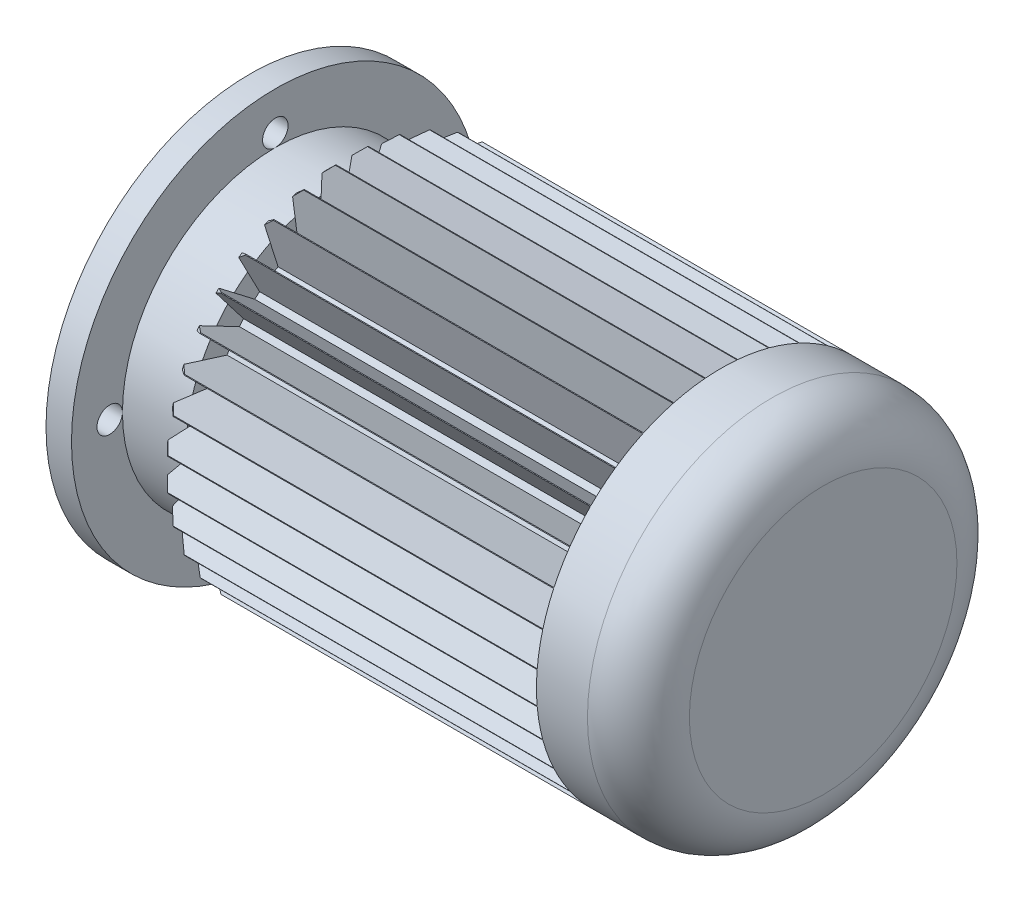
SolidWorks part; units mm, degrees
ref_plane "前视基准面" through (0, 0, 0) normal (0, 0, 1) x (1, 0, 0)
ref_plane "上视基准面" through (0, 0, 0) normal (0, 1, 0) x (1, 0, 0)
ref_plane "右视基准面" through (0, 0, 0) normal (1, 0, 0) x (0, 0, -1)
sketch "草图1" plane through (0, 0, 0) normal (0, 0, 1) x (1, 0, 0)
  line L0 (0, 0) -> (197.0687, 0) construction
  line L1 (0, 0) -> (0, 55)
  line L2 (0, -55) -> (0, 55) construction
  line L3 (0, 55) -> (3.5, 55)
  line L4 (3.5, 55) -> (3.5, 80)
  line L5 (3.5, 80) -> (13.5, 80)
  line L6 (13.5, 80) -> (13.5, 60)
  line L7 (13.5, 60) -> (38.5, 60)
  line L8 (38.5, 60) -> (38.5, 72.5)
  line L9 (38.5, 72.5) -> (228.5, 72.5)
  line L10 (228.5, 72.5) -> (228.5, 0)
  line L11 (55, 0) -> (-55, 0) construction
  line L12 (0, 0) -> (228.5, 0)
  dimension "D1" = 55
  dimension "D2" = 80
  dimension "D3" = 3.5
  dimension "D4" = 10
  dimension "D5" = 225
  dimension "D6" = 72.5
  dimension "D7" = 25
  dimension "D8" = 60
revolve "旋转1" add sketch "草图1" angle 360 about L0
fillet "圆角1" radius 20 1 edges at (228.5, 0, 72.5)
chamfer "倒角1" distance 5 angle 45 1 edges at (38.5, 0, 72.5)
sketch "草图3" plane through (38.5, 0, 0) normal (-1, 0, 0) x (0, 0, 1)
  line L0 (6.1796, 72.2362) -> (1.25, 50)
  line L1 (0, -55) -> (0, 55) construction
  line L2 (0, 0) -> (0, 72.5) construction
  line L3 (55, 0) -> (-55, 0) construction
  line L4 (-6.1796, 72.2362) -> (-1.25, 50)
  line L5 (-1.25, 50) -> (1.25, 50)
  line L6 (0, 67.0138) -> (0, 78.2835) construction
  circle A0 centre (0, 0) radius 72.5 construction
  arc A1 (6.1796, 72.2362) -> (-6.1796, 72.2362) centre (0, 0) ccw
  dimension "D1" = 1.25
  dimension "D2" = 50
  dimension "D3" = 12.5
  dimension "D4" = 12.5
extrude "切除-拉伸1" cut sketch "草图3" against normal blind 150
pattern_circular "阵列(圆周)1" count 36 every 10 about axis through (0, 0, 0) along (1, 0, 0) of "切除-拉伸1"
sketch "草图4" plane through (3.5, 0, 0) normal (-1, 0, 0) x (0, 0, 1)
  line L0 (0, -88) -> (0, 88) construction
  line L1 (88, 0) -> (-88, 0) construction
  circle A0 centre (0, 65) radius 5
  dimension "D1" = 10
  dimension "D2" = 65
extrude "切除-拉伸2" cut sketch "草图4" against normal up to next
pattern_circular "阵列(圆周)2" count 4 every 90 about axis through (0, 0, 0) along (1, 0, 0) of "切除-拉伸2"
